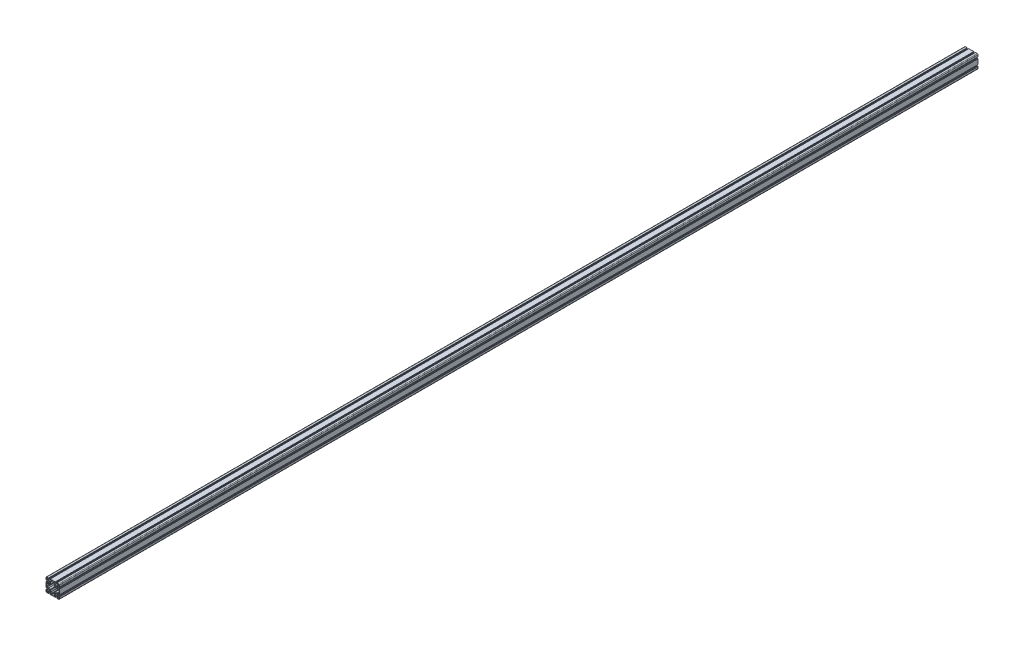
SolidWorks part; units mm, degrees
ref_plane "Front Plane" through (0, 0, 0) normal (0, 0, 1) x (1, 0, 0)
ref_plane "Top Plane" through (0, 0, 0) normal (0, 1, 0) x (1, 0, 0)
ref_plane "Right Plane" through (0, 0, 0) normal (1, 0, 0) x (0, 0, -1)
ref_plane "Plane1" through (0, 0, 100) normal (0, 0, 1) x (1, 0, 0)
sketch "Sketch1" plane through (0, 0, 100) normal (0, 0, 1) x (1, 0, 0)
  line L0 (-29.6117, 8.4562) -> (-25.1475, 12.9204)
  line L1 (-25.1475, 12.9204) -> (-14.0153, 12.9204)
  line L2 (-11.5153, 15.4204) -> (-11.5153, 26.5526)
  line L3 (-11.5153, 26.5526) -> (-7.0511, 31.0168)
  line L4 (-6.4653, 32.4311) -> (-6.4653, 37.4204)
  line L5 (-5.4653, 38.4204) -> (7.0347, 38.4204)
  line L6 (8.0347, 37.4204) -> (8.0347, 32.4311)
  line L7 (8.6205, 31.0168) -> (13.0847, 26.5526)
  line L8 (13.0847, 26.5526) -> (13.0847, 15.4204)
  line L9 (15.5847, 12.9204) -> (26.717, 12.9204)
  line L10 (26.717, 12.9204) -> (31.1812, 8.4562)
  line L11 (32.5954, 7.8704) -> (37.5847, 7.8704)
  line L12 (38.5847, 6.8704) -> (38.5847, -5.6296)
  line L13 (37.5847, -6.6296) -> (32.5954, -6.6296)
  line L14 (31.1812, -7.2154) -> (26.717, -11.6796)
  line L15 (26.717, -11.6796) -> (15.5847, -11.6796)
  line L16 (13.0847, -14.1796) -> (13.0847, -24.4834)
  line L17 (12.4989, -25.8976) -> (8.6205, -29.776)
  line L18 (8.0347, -31.1903) -> (8.0347, -36.1796)
  line L19 (7.0347, -37.1796) -> (-5.4653, -37.1796)
  line L20 (-6.4653, -36.1796) -> (-6.4653, -31.1903)
  line L21 (-7.0511, -29.776) -> (-11.5153, -25.3118)
  line L22 (-11.5153, -25.3118) -> (-11.5153, -14.1796)
  line L23 (-14.0153, -11.6796) -> (-25.1475, -11.6796)
  line L24 (-25.1475, -11.6796) -> (-29.6117, -7.2154)
  line L25 (-31.0259, -6.6296) -> (-36.0153, -6.6296)
  line L26 (-37.0153, -5.6296) -> (-37.0153, 6.8704)
  line L27 (-36.0153, 7.8704) -> (-31.0259, 7.8704)
  line L28 (-35.2193, 39.1244) -> (-31.9653, 39.1244)
  line L29 (-30.9653, 38.1244) -> (-30.9653, 33.3704)
  line L30 (-31.9653, 32.3704) -> (-36.7193, 32.3704)
  line L31 (-37.7193, 33.3704) -> (-37.7193, 36.6244)
  line L32 (36.7887, -37.8836) -> (33.5347, -37.8836)
  line L33 (32.5347, -36.8836) -> (32.5347, -32.1296)
  line L34 (33.5347, -31.1296) -> (38.2887, -31.1296)
  line L35 (39.2887, -32.1296) -> (39.2887, -35.3836)
  line L36 (37.7847, 10.3704) -> (32.8025, 10.3704)
  line L37 (32.8025, 10.3704) -> (28.4847, 14.6882)
  line L38 (28.4847, 14.6882) -> (28.4847, 26.5526)
  line L39 (28.4847, 26.5526) -> (32.8025, 30.8704)
  line L40 (32.8025, 30.8704) -> (37.7847, 30.8704)
  line L41 (38.7847, 29.8704) -> (38.7847, 28.2204)
  line L42 (37.7847, 27.2204) -> (36.2847, 27.2204)
  line L43 (36.2847, 27.2204) -> (36.2847, 25.0204)
  line L44 (36.5847, 24.7204) -> (39.7847, 24.7204)
  line L45 (39.7847, 24.7204) -> (39.7847, 25.5204)
  line L46 (39.9847, 25.7204) -> (40.7847, 25.7204)
  line L47 (40.7847, 25.7204) -> (40.7847, 36.1204)
  line L48 (36.2847, 40.6204) -> (25.8847, 40.6204)
  line L49 (25.8847, 40.6204) -> (25.8847, 39.8204)
  line L50 (25.6847, 39.6204) -> (24.8847, 39.6204)
  line L51 (24.8847, 39.6204) -> (24.8847, 36.4204)
  line L52 (25.1847, 36.1204) -> (27.3847, 36.1204)
  line L53 (27.3847, 36.1204) -> (27.3847, 37.6204)
  line L54 (28.3847, 38.6204) -> (30.0347, 38.6204)
  line L55 (31.0347, 37.6204) -> (31.0347, 32.6382)
  line L56 (31.0347, 32.6382) -> (26.717, 28.3204)
  line L57 (26.717, 28.3204) -> (14.8525, 28.3204)
  line L58 (14.8525, 28.3204) -> (10.5347, 32.6382)
  line L59 (10.5347, 32.6382) -> (10.5347, 37.6204)
  line L60 (11.5347, 38.6204) -> (13.1847, 38.6204)
  line L61 (14.1847, 37.6204) -> (14.1847, 36.1204)
  line L62 (14.1847, 36.1204) -> (16.3847, 36.1204)
  line L63 (16.6847, 36.4204) -> (16.6847, 39.6204)
  line L64 (16.6847, 39.6204) -> (15.8847, 39.6204)
  line L65 (15.6847, 39.8204) -> (15.6847, 40.6204)
  line L66 (15.6847, 40.6204) -> (-14.1153, 40.6204)
  line L67 (-14.1153, 40.6204) -> (-14.1153, 39.8204)
  line L68 (-14.3153, 39.6204) -> (-15.1153, 39.6204)
  line L69 (-15.1153, 39.6204) -> (-15.1153, 36.4204)
  line L70 (-14.8153, 36.1204) -> (-12.6153, 36.1204)
  line L71 (-12.6153, 36.1204) -> (-12.6153, 37.6204)
  line L72 (-11.6153, 38.6204) -> (-9.9653, 38.6204)
  line L73 (-8.9653, 37.6204) -> (-8.9653, 32.6382)
  line L74 (-8.9653, 32.6382) -> (-13.283, 28.3204)
  line L75 (-13.283, 28.3204) -> (-25.1475, 28.3204)
  line L76 (-25.1475, 28.3204) -> (-29.4653, 32.6382)
  line L77 (-29.4653, 32.6382) -> (-29.4653, 37.6204)
  line L78 (-28.4653, 38.6204) -> (-26.8153, 38.6204)
  line L79 (-25.8153, 37.6204) -> (-25.8153, 36.1204)
  line L80 (-25.8153, 36.1204) -> (-23.6153, 36.1204)
  line L81 (-23.3153, 36.4204) -> (-23.3153, 39.6204)
  line L82 (-23.3153, 39.6204) -> (-24.1153, 39.6204)
  line L83 (-24.3153, 39.8204) -> (-24.3153, 40.6204)
  line L84 (-24.3153, 40.6204) -> (-34.7153, 40.6204)
  line L85 (-39.2153, 36.1204) -> (-39.2153, 25.7204)
  line L86 (-39.2153, 25.7204) -> (-38.4153, 25.7204)
  line L87 (-38.2153, 25.5204) -> (-38.2153, 24.7204)
  line L88 (-38.2153, 24.7204) -> (-35.0153, 24.7204)
  line L89 (-34.7153, 25.0204) -> (-34.7153, 27.2204)
  line L90 (-34.7153, 27.2204) -> (-36.2153, 27.2204)
  line L91 (-37.2153, 28.2204) -> (-37.2153, 29.8704)
  line L92 (-36.2153, 30.8704) -> (-31.233, 30.8704)
  line L93 (-31.233, 30.8704) -> (-26.9153, 26.5526)
  line L94 (-26.9153, 26.5526) -> (-26.9153, 14.6882)
  line L95 (-26.9153, 14.6882) -> (-31.233, 10.3704)
  line L96 (-31.233, 10.3704) -> (-36.2153, 10.3704)
  line L97 (-37.2153, 11.3704) -> (-37.2153, 13.0204)
  line L98 (-36.2153, 14.0204) -> (-34.7153, 14.0204)
  line L99 (-34.7153, 14.0204) -> (-34.7153, 16.2204)
  line L100 (-35.0153, 16.5204) -> (-38.2153, 16.5204)
  line L101 (-38.2153, 16.5204) -> (-38.2153, 15.7204)
  line L102 (-38.4153, 15.5204) -> (-39.2153, 15.5204)
  line L103 (-39.2153, 15.5204) -> (-39.2153, -14.2796)
  line L104 (-39.2153, -14.2796) -> (-38.4153, -14.2796)
  line L105 (-38.2153, -14.4796) -> (-38.2153, -15.2796)
  line L106 (-38.2153, -15.2796) -> (-35.0153, -15.2796)
  line L107 (-34.7153, -14.9796) -> (-34.7153, -12.7796)
  line L108 (-34.7153, -12.7796) -> (-36.2153, -12.7796)
  line L109 (-37.2153, -11.7796) -> (-37.2153, -10.1296)
  line L110 (-36.2153, -9.1296) -> (-31.233, -9.1296)
  line L111 (-31.233, -9.1296) -> (-26.9153, -13.4474)
  line L112 (-26.9153, -13.4474) -> (-26.9153, -25.3118)
  line L113 (-26.9153, -25.3118) -> (-31.233, -29.6296)
  line L114 (-31.233, -29.6296) -> (-36.2153, -29.6296)
  line L115 (-37.2153, -28.6296) -> (-37.2153, -26.9796)
  line L116 (-36.2153, -25.9796) -> (-34.7153, -25.9796)
  line L117 (-34.7153, -25.9796) -> (-34.7153, -23.7796)
  line L118 (-35.0153, -23.4796) -> (-38.2153, -23.4796)
  line L119 (-38.2153, -23.4796) -> (-38.2153, -24.2796)
  line L120 (-38.4153, -24.4796) -> (-39.2153, -24.4796)
  line L121 (-39.2153, -24.4796) -> (-39.2153, -34.8796)
  line L122 (-34.7153, -39.3796) -> (-24.3153, -39.3796)
  line L123 (-24.3153, -39.3796) -> (-24.3153, -38.5796)
  line L124 (-24.1153, -38.3796) -> (-23.3153, -38.3796)
  line L125 (-23.3153, -38.3796) -> (-23.3153, -35.1796)
  line L126 (-23.6153, -34.8796) -> (-25.8153, -34.8796)
  line L127 (-25.8153, -34.8796) -> (-25.8153, -36.3796)
  line L128 (-26.8153, -37.3796) -> (-28.4653, -37.3796)
  line L129 (-29.4653, -36.3796) -> (-29.4653, -31.3974)
  line L130 (-29.4653, -31.3974) -> (-25.1475, -27.0796)
  line L131 (-25.1475, -27.0796) -> (-13.283, -27.0796)
  line L132 (-13.283, -27.0796) -> (-8.9653, -31.3974)
  line L133 (-8.9653, -31.3974) -> (-8.9653, -36.3796)
  line L134 (-9.9653, -37.3796) -> (-11.6153, -37.3796)
  line L135 (-12.6153, -36.3796) -> (-12.6153, -34.8796)
  line L136 (-12.6153, -34.8796) -> (-14.8153, -34.8796)
  line L137 (-15.1153, -35.1796) -> (-15.1153, -38.3796)
  line L138 (-15.1153, -38.3796) -> (-14.3153, -38.3796)
  line L139 (-14.1153, -38.5796) -> (-14.1153, -39.3796)
  line L140 (-14.1153, -39.3796) -> (15.6847, -39.3796)
  line L141 (15.6847, -39.3796) -> (15.6847, -38.5796)
  line L142 (15.8847, -38.3796) -> (16.6847, -38.3796)
  line L143 (16.6847, -38.3796) -> (16.6847, -35.1796)
  line L144 (16.3847, -34.8796) -> (14.1847, -34.8796)
  line L145 (14.1847, -34.8796) -> (14.1847, -36.3796)
  line L146 (13.1847, -37.3796) -> (11.5347, -37.3796)
  line L147 (10.5347, -36.3796) -> (10.5347, -31.3974)
  line L148 (10.5347, -31.3974) -> (14.8525, -27.0796)
  line L149 (14.8525, -27.0796) -> (26.717, -27.0796)
  line L150 (26.717, -27.0796) -> (31.0347, -31.3974)
  line L151 (31.0347, -31.3974) -> (31.0347, -36.3796)
  line L152 (30.0347, -37.3796) -> (28.3847, -37.3796)
  line L153 (27.3847, -36.3796) -> (27.3847, -34.8796)
  line L154 (27.3847, -34.8796) -> (25.1847, -34.8796)
  line L155 (24.8847, -35.1796) -> (24.8847, -38.3796)
  line L156 (24.8847, -38.3796) -> (25.6847, -38.3796)
  line L157 (25.8847, -38.5796) -> (25.8847, -39.3796)
  line L158 (25.8847, -39.3796) -> (36.2847, -39.3796)
  line L159 (40.7847, -34.8796) -> (40.7847, -24.4796)
  line L160 (40.7847, -24.4796) -> (39.9847, -24.4796)
  line L161 (39.7847, -24.2796) -> (39.7847, -23.4796)
  line L162 (39.7847, -23.4796) -> (36.5847, -23.4796)
  line L163 (36.2847, -23.7796) -> (36.2847, -25.9796)
  line L164 (36.2847, -25.9796) -> (37.7847, -25.9796)
  line L165 (38.7847, -26.9796) -> (38.7847, -28.6296)
  line L166 (37.7847, -29.6296) -> (32.8025, -29.6296)
  line L167 (32.8025, -29.6296) -> (28.4847, -25.3118)
  line L168 (28.4847, -25.3118) -> (28.4847, -13.4474)
  line L169 (28.4847, -13.4474) -> (32.8025, -9.1296)
  line L170 (32.8025, -9.1296) -> (37.7847, -9.1296)
  line L171 (38.7847, -10.1296) -> (38.7847, -11.7796)
  line L172 (37.7847, -12.7796) -> (36.2847, -12.7796)
  line L173 (36.2847, -12.7796) -> (36.2847, -14.9796)
  line L174 (36.5847, -15.2796) -> (39.7847, -15.2796)
  line L175 (39.7847, -15.2796) -> (39.7847, -14.4796)
  line L176 (39.9847, -14.2796) -> (40.7847, -14.2796)
  line L177 (40.7847, -14.2796) -> (40.7847, 15.5204)
  line L178 (40.7847, 15.5204) -> (39.9847, 15.5204)
  line L179 (39.7847, 15.7204) -> (39.7847, 16.5204)
  line L180 (39.7847, 16.5204) -> (36.5847, 16.5204)
  line L181 (36.2847, 16.2204) -> (36.2847, 14.0204)
  line L182 (36.2847, 14.0204) -> (37.7847, 14.0204)
  line L183 (38.7847, 13.0204) -> (38.7847, 11.3704)
  line L184 (-37.7193, -35.3836) -> (-37.7193, -32.1296)
  line L185 (-36.7193, -31.1296) -> (-31.9653, -31.1296)
  line L186 (-30.9653, -32.1296) -> (-30.9653, -36.8836)
  line L187 (-31.9653, -37.8836) -> (-35.2193, -37.8836)
  line L188 (39.2887, 36.6244) -> (39.2887, 33.3704)
  line L189 (38.2887, 32.3704) -> (33.5347, 32.3704)
  line L190 (32.5347, 33.3704) -> (32.5347, 38.1244)
  line L191 (33.5347, 39.1244) -> (36.7887, 39.1244)
  arc A0 (-14.0153, 12.9204) -> (-11.5153, 15.4204) centre (-14.0153, 15.4204) ccw
  arc A1 (-7.0511, 31.0168) -> (-6.4653, 32.4311) centre (-8.4653, 32.4311) ccw
  arc A2 (-6.4653, 37.4204) -> (-5.4653, 38.4204) centre (-5.4653, 37.4204) cw
  arc A3 (7.0347, 38.4204) -> (8.0347, 37.4204) centre (7.0347, 37.4204) cw
  arc A4 (8.0347, 32.4311) -> (8.6205, 31.0168) centre (10.0347, 32.4311) ccw
  arc A5 (13.0847, 15.4204) -> (15.5847, 12.9204) centre (15.5847, 15.4204) ccw
  arc A6 (31.1812, 8.4562) -> (32.5954, 7.8704) centre (32.5954, 9.8704) ccw
  arc A7 (37.5847, 7.8704) -> (38.5847, 6.8704) centre (37.5847, 6.8704) cw
  arc A8 (38.5847, -5.6296) -> (37.5847, -6.6296) centre (37.5847, -5.6296) cw
  arc A9 (32.5954, -6.6296) -> (31.1812, -7.2154) centre (32.5954, -8.6296) ccw
  arc A10 (15.5847, -11.6796) -> (13.0847, -14.1796) centre (15.5847, -14.1796) ccw
  arc A11 (13.0847, -24.4834) -> (12.4989, -25.8976) centre (11.0847, -24.4834) cw
  arc A12 (8.6205, -29.776) -> (8.0347, -31.1903) centre (10.0347, -31.1903) ccw
  arc A13 (8.0347, -36.1796) -> (7.0347, -37.1796) centre (7.0347, -36.1796) cw
  arc A14 (-5.4653, -37.1796) -> (-6.4653, -36.1796) centre (-5.4653, -36.1796) cw
  arc A15 (-6.4653, -31.1903) -> (-7.0511, -29.776) centre (-8.4653, -31.1903) ccw
  arc A16 (-11.5153, -14.1796) -> (-14.0153, -11.6796) centre (-14.0153, -14.1796) ccw
  arc A17 (-29.6117, -7.2154) -> (-31.0259, -6.6296) centre (-31.0259, -8.6296) ccw
  arc A18 (-36.0153, -6.6296) -> (-37.0153, -5.6296) centre (-36.0153, -5.6296) cw
  arc A19 (-37.0153, 6.8704) -> (-36.0153, 7.8704) centre (-36.0153, 6.8704) cw
  arc A20 (-31.0259, 7.8704) -> (-29.6117, 8.4562) centre (-31.0259, 9.8704) ccw
  arc A21 (-31.9653, 39.1244) -> (-30.9653, 38.1244) centre (-31.9653, 38.1244) cw
  arc A22 (-30.9653, 33.3704) -> (-31.9653, 32.3704) centre (-31.9653, 33.3704) cw
  arc A23 (-36.7193, 32.3704) -> (-37.7193, 33.3704) centre (-36.7193, 33.3704) cw
  arc A24 (-37.7193, 36.6244) -> (-35.2193, 39.1244) centre (-35.2193, 36.6244) cw
  circle A25 centre (-19.2153, -19.3796) radius 3.4
  circle A26 centre (20.7847, -19.3796) radius 3.4
  arc A27 (33.5347, -37.8836) -> (32.5347, -36.8836) centre (33.5347, -36.8836) cw
  arc A28 (32.5347, -32.1296) -> (33.5347, -31.1296) centre (33.5347, -32.1296) cw
  arc A29 (38.2887, -31.1296) -> (39.2887, -32.1296) centre (38.2887, -32.1296) cw
  arc A30 (39.2887, -35.3836) -> (36.7887, -37.8836) centre (36.7887, -35.3836) cw
  arc A31 (37.7847, 30.8704) -> (38.7847, 29.8704) centre (37.7847, 29.8704) cw
  arc A32 (38.7847, 28.2204) -> (37.7847, 27.2204) centre (37.7847, 28.2204) cw
  arc A33 (36.2847, 25.0204) -> (36.5847, 24.7204) centre (36.5847, 25.0204) ccw
  arc A34 (39.7847, 25.5204) -> (39.9847, 25.7204) centre (39.9847, 25.5204) cw
  arc A35 (40.7847, 36.1204) -> (36.2847, 40.6204) centre (36.2847, 36.1204) ccw
  arc A36 (25.8847, 39.8204) -> (25.6847, 39.6204) centre (25.6847, 39.8204) cw
  arc A37 (24.8847, 36.4204) -> (25.1847, 36.1204) centre (25.1847, 36.4204) ccw
  arc A38 (27.3847, 37.6204) -> (28.3847, 38.6204) centre (28.3847, 37.6204) cw
  arc A39 (30.0347, 38.6204) -> (31.0347, 37.6204) centre (30.0347, 37.6204) cw
  arc A40 (10.5347, 37.6204) -> (11.5347, 38.6204) centre (11.5347, 37.6204) cw
  arc A41 (13.1847, 38.6204) -> (14.1847, 37.6204) centre (13.1847, 37.6204) cw
  arc A42 (16.3847, 36.1204) -> (16.6847, 36.4204) centre (16.3847, 36.4204) ccw
  arc A43 (15.8847, 39.6204) -> (15.6847, 39.8204) centre (15.8847, 39.8204) cw
  arc A44 (-14.1153, 39.8204) -> (-14.3153, 39.6204) centre (-14.3153, 39.8204) cw
  arc A45 (-15.1153, 36.4204) -> (-14.8153, 36.1204) centre (-14.8153, 36.4204) ccw
  arc A46 (-12.6153, 37.6204) -> (-11.6153, 38.6204) centre (-11.6153, 37.6204) cw
  arc A47 (-9.9653, 38.6204) -> (-8.9653, 37.6204) centre (-9.9653, 37.6204) cw
  arc A48 (-29.4653, 37.6204) -> (-28.4653, 38.6204) centre (-28.4653, 37.6204) cw
  arc A49 (-26.8153, 38.6204) -> (-25.8153, 37.6204) centre (-26.8153, 37.6204) cw
  arc A50 (-23.6153, 36.1204) -> (-23.3153, 36.4204) centre (-23.6153, 36.4204) ccw
  arc A51 (-24.1153, 39.6204) -> (-24.3153, 39.8204) centre (-24.1153, 39.8204) cw
  arc A52 (-34.7153, 40.6204) -> (-39.2153, 36.1204) centre (-34.7153, 36.1204) ccw
  arc A53 (-38.4153, 25.7204) -> (-38.2153, 25.5204) centre (-38.4153, 25.5204) cw
  arc A54 (-35.0153, 24.7204) -> (-34.7153, 25.0204) centre (-35.0153, 25.0204) ccw
  arc A55 (-36.2153, 27.2204) -> (-37.2153, 28.2204) centre (-36.2153, 28.2204) cw
  arc A56 (-37.2153, 29.8704) -> (-36.2153, 30.8704) centre (-36.2153, 29.8704) cw
  arc A57 (-36.2153, 10.3704) -> (-37.2153, 11.3704) centre (-36.2153, 11.3704) cw
  arc A58 (-37.2153, 13.0204) -> (-36.2153, 14.0204) centre (-36.2153, 13.0204) cw
  arc A59 (-34.7153, 16.2204) -> (-35.0153, 16.5204) centre (-35.0153, 16.2204) ccw
  arc A60 (-38.2153, 15.7204) -> (-38.4153, 15.5204) centre (-38.4153, 15.7204) cw
  arc A61 (-38.4153, -14.2796) -> (-38.2153, -14.4796) centre (-38.4153, -14.4796) cw
  arc A62 (-35.0153, -15.2796) -> (-34.7153, -14.9796) centre (-35.0153, -14.9796) ccw
  arc A63 (-36.2153, -12.7796) -> (-37.2153, -11.7796) centre (-36.2153, -11.7796) cw
  arc A64 (-37.2153, -10.1296) -> (-36.2153, -9.1296) centre (-36.2153, -10.1296) cw
  arc A65 (-36.2153, -29.6296) -> (-37.2153, -28.6296) centre (-36.2153, -28.6296) cw
  arc A66 (-37.2153, -26.9796) -> (-36.2153, -25.9796) centre (-36.2153, -26.9796) cw
  arc A67 (-34.7153, -23.7796) -> (-35.0153, -23.4796) centre (-35.0153, -23.7796) ccw
  arc A68 (-38.2153, -24.2796) -> (-38.4153, -24.4796) centre (-38.4153, -24.2796) cw
  arc A69 (-39.2153, -34.8796) -> (-34.7153, -39.3796) centre (-34.7153, -34.8796) ccw
  arc A70 (-24.3153, -38.5796) -> (-24.1153, -38.3796) centre (-24.1153, -38.5796) cw
  arc A71 (-23.3153, -35.1796) -> (-23.6153, -34.8796) centre (-23.6153, -35.1796) ccw
  arc A72 (-25.8153, -36.3796) -> (-26.8153, -37.3796) centre (-26.8153, -36.3796) cw
  arc A73 (-28.4653, -37.3796) -> (-29.4653, -36.3796) centre (-28.4653, -36.3796) cw
  arc A74 (-8.9653, -36.3796) -> (-9.9653, -37.3796) centre (-9.9653, -36.3796) cw
  arc A75 (-11.6153, -37.3796) -> (-12.6153, -36.3796) centre (-11.6153, -36.3796) cw
  arc A76 (-14.8153, -34.8796) -> (-15.1153, -35.1796) centre (-14.8153, -35.1796) ccw
  arc A77 (-14.3153, -38.3796) -> (-14.1153, -38.5796) centre (-14.3153, -38.5796) cw
  arc A78 (15.6847, -38.5796) -> (15.8847, -38.3796) centre (15.8847, -38.5796) cw
  arc A79 (16.6847, -35.1796) -> (16.3847, -34.8796) centre (16.3847, -35.1796) ccw
  arc A80 (14.1847, -36.3796) -> (13.1847, -37.3796) centre (13.1847, -36.3796) cw
  arc A81 (11.5347, -37.3796) -> (10.5347, -36.3796) centre (11.5347, -36.3796) cw
  arc A82 (31.0347, -36.3796) -> (30.0347, -37.3796) centre (30.0347, -36.3796) cw
  arc A83 (28.3847, -37.3796) -> (27.3847, -36.3796) centre (28.3847, -36.3796) cw
  arc A84 (25.1847, -34.8796) -> (24.8847, -35.1796) centre (25.1847, -35.1796) ccw
  arc A85 (25.6847, -38.3796) -> (25.8847, -38.5796) centre (25.6847, -38.5796) cw
  arc A86 (36.2847, -39.3796) -> (40.7847, -34.8796) centre (36.2847, -34.8796) ccw
  arc A87 (39.9847, -24.4796) -> (39.7847, -24.2796) centre (39.9847, -24.2796) cw
  arc A88 (36.5847, -23.4796) -> (36.2847, -23.7796) centre (36.5847, -23.7796) ccw
  arc A89 (37.7847, -25.9796) -> (38.7847, -26.9796) centre (37.7847, -26.9796) cw
  arc A90 (38.7847, -28.6296) -> (37.7847, -29.6296) centre (37.7847, -28.6296) cw
  arc A91 (37.7847, -9.1296) -> (38.7847, -10.1296) centre (37.7847, -10.1296) cw
  arc A92 (38.7847, -11.7796) -> (37.7847, -12.7796) centre (37.7847, -11.7796) cw
  arc A93 (36.2847, -14.9796) -> (36.5847, -15.2796) centre (36.5847, -14.9796) ccw
  arc A94 (39.7847, -14.4796) -> (39.9847, -14.2796) centre (39.9847, -14.4796) cw
  arc A95 (39.9847, 15.5204) -> (39.7847, 15.7204) centre (39.9847, 15.7204) cw
  arc A96 (36.5847, 16.5204) -> (36.2847, 16.2204) centre (36.5847, 16.2204) ccw
  arc A97 (37.7847, 14.0204) -> (38.7847, 13.0204) centre (37.7847, 13.0204) cw
  arc A98 (38.7847, 11.3704) -> (37.7847, 10.3704) centre (37.7847, 11.3704) cw
  arc A99 (-37.7193, -32.1296) -> (-36.7193, -31.1296) centre (-36.7193, -32.1296) cw
  arc A100 (-31.9653, -31.1296) -> (-30.9653, -32.1296) centre (-31.9653, -32.1296) cw
  arc A101 (-30.9653, -36.8836) -> (-31.9653, -37.8836) centre (-31.9653, -36.8836) cw
  arc A102 (-35.2193, -37.8836) -> (-37.7193, -35.3836) centre (-35.2193, -35.3836) cw
  arc A103 (39.2887, 33.3704) -> (38.2887, 32.3704) centre (38.2887, 33.3704) cw
  arc A104 (33.5347, 32.3704) -> (32.5347, 33.3704) centre (33.5347, 33.3704) cw
  arc A105 (32.5347, 38.1244) -> (33.5347, 39.1244) centre (33.5347, 38.1244) cw
  arc A106 (36.7887, 39.1244) -> (39.2887, 36.6244) centre (36.7887, 36.6244) cw
  circle A107 centre (20.7847, 20.6204) radius 3.4
  circle A108 centre (-19.2153, 20.6204) radius 3.4
extrude "Boss-Extrude1" add sketch "Sketch1" against normal blind 5500
